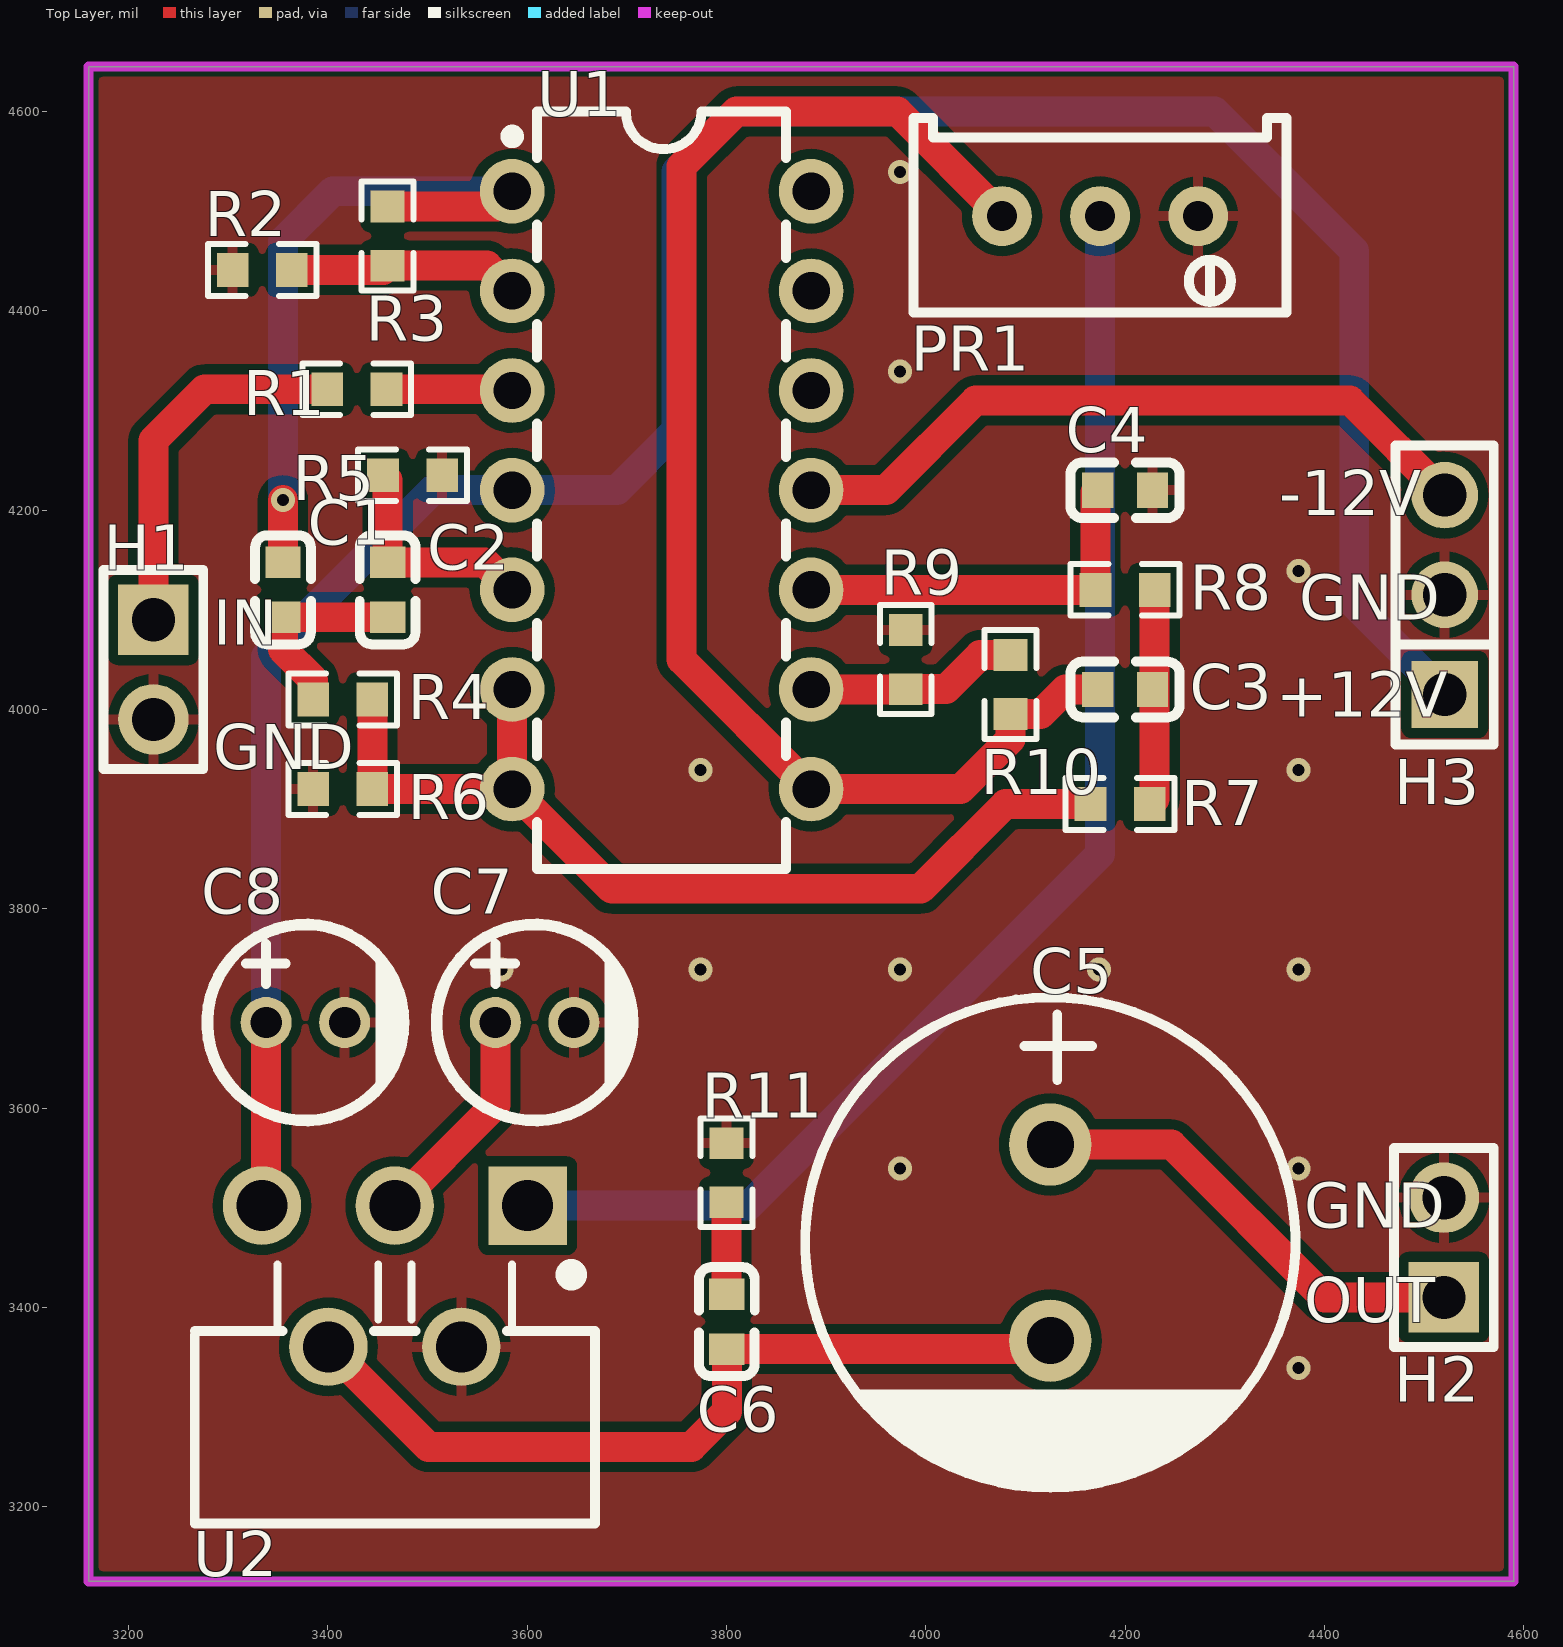
[diagram p0: Top Layer view]
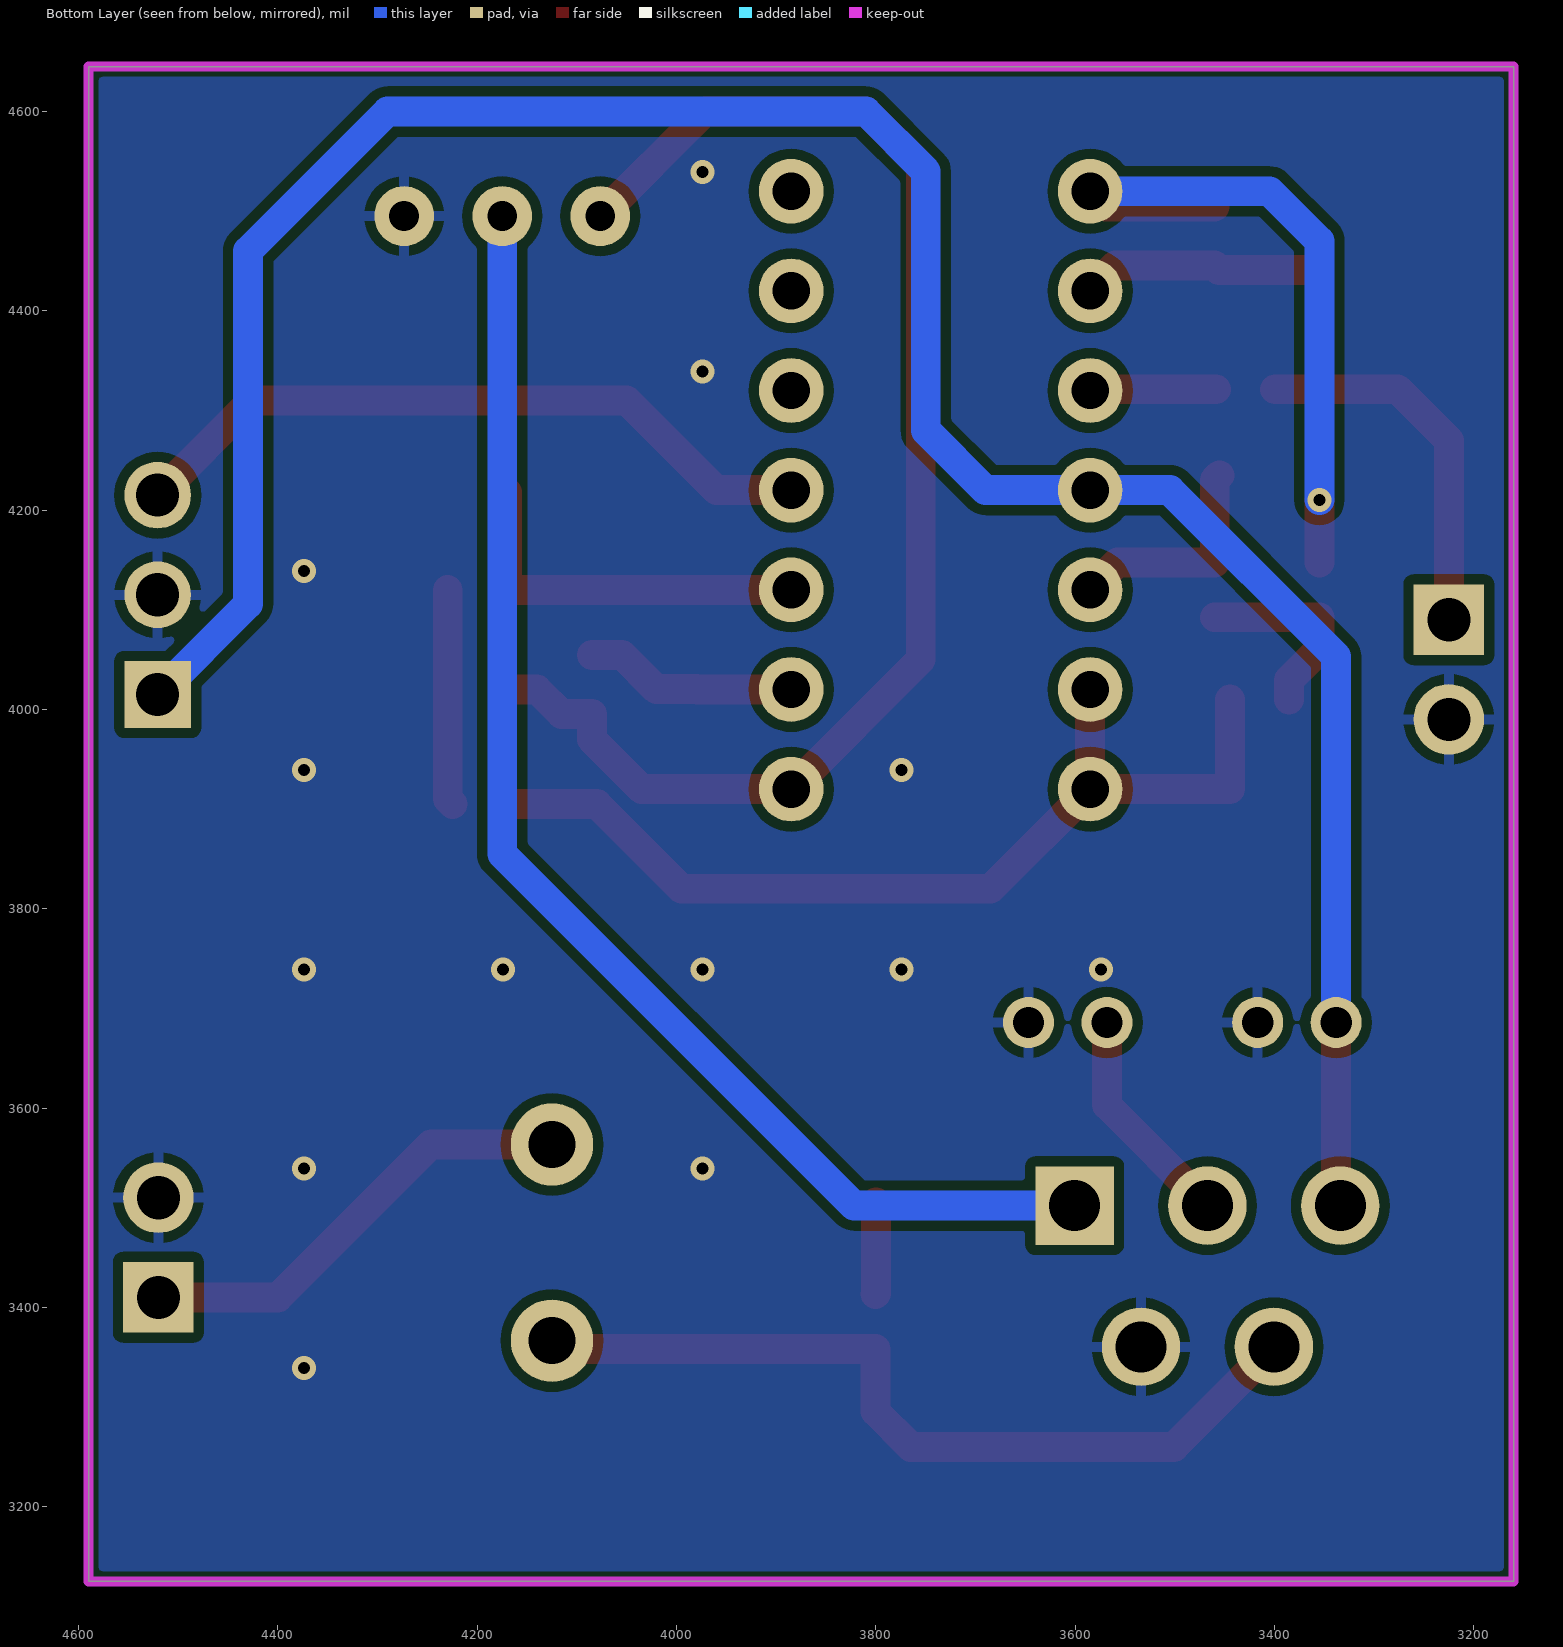
[diagram p1: Bottom Layer view, seen from below]
# Altium PCB MISC49872.pcbdoc
Units mil, origin at the board's own origin, x right, y up, seen from the top; angles counter-clockwise.
Board outline 1430 x 1520 mil, 2 copper layers (Top Layer, Bottom Layer), stack 62.206 mil thick; 25 components, 19 nets, 67 pads, 14 vias.

## Layer stack, top to bottom
Top Solder Mask Layer: solder mask 0.394, Dk 3.3
Top Layer: signal copper 1.379
Dielectric1: surface 59.449, FR4, Dk 4.5
Bottom Layer: signal copper 1.378
Bottom Solder Mask Layer: solder mask 0.394, Dk 3.3

## Board outline
3160,4645 3160,3125 4590,3125 4590,4645

## Design rules (kind name [scope] priority, off if disabled: settings)
BoardOutlineClearance copperThickness2oz_1 [All] p2 off: genericclearance=7.99 ignorepadtopadclearanceinfootprint=FALSE except(0: Arc-SplitContinuation Track-SplitContinuation SMDPad-SplitContinuation THPad-SplitContinuation Via-SplitContinuation Fill-SplitContinuation Region-SplitContinuation Poly-SplitContinuation Text-SplitContinuation Hole-SplitContinuation; 5.98: Arc-CutoutEdge SMDPad-CutoutEdge THPad-CutoutEdge Via-CutoutEdge Fill-CutoutEdge Region-CutoutEdge Text-CutoutEdge; 6.93: Hole-OutlineEdge Hole-CutoutEdge; 10: Poly-OutlineEdge Poly-CutoutEdge; 11.81: Arc-OutlineEdge Track-OutlineEdge SMDPad-OutlineEdge THPad-OutlineEdge Via-OutlineEdge Fill-OutlineEdge Region-OutlineEdge Text-OutlineEdge Track-CutoutEdge)
BoardOutlineClearance copperThickness1oz_1 [All] p4: genericclearance=4.02 ignorepadtopadclearanceinfootprint=FALSE except(0: Arc-SplitContinuation Track-SplitContinuation SMDPad-SplitContinuation THPad-SplitContinuation Via-SplitContinuation Fill-SplitContinuation Region-SplitContinuation Poly-SplitContinuation Text-SplitContinuation Hole-SplitContinuation; 6: SMDPad-CutoutEdge THPad-CutoutEdge Via-CutoutEdge Fill-CutoutEdge Region-CutoutEdge Text-CutoutEdge; 6.93: Hole-OutlineEdge Hole-CutoutEdge; 10: Poly-OutlineEdge Poly-CutoutEdge; 11.8: Arc-OutlineEdge Track-OutlineEdge SMDPad-OutlineEdge THPad-OutlineEdge Via-OutlineEdge Fill-OutlineEdge Region-OutlineEdge Text-OutlineEdge; 11.81: Arc-CutoutEdge Track-CutoutEdge)
Clearance copperThickness2oz [All] p1 off: gap=7.99 ignorepadtopadclearanceinfootprint=FALSE except(5.98: SMDPad-Track SMDPad-SMDPad THPad-Track SMDPad-THPad THPad-THPad Track-Via SMDPad-Via THPad-Via Via-Via Fill-Track Region-Track Fill-SMDPad Region-SMDPad Fill-THPad Region-THPad Fill-Via Region-Via Fill-Fill Fill-Region Region-Region Arc-Track Arc-SMDPad Arc-THPad Arc-Via Fill-Arc Region-Arc Arc-Arc Text-Track SMDPad-Text Text-THPad Text-Via Fill-Text Region-Text Arc-Text Text-Text; 6.93: Hole-Track Hole-SMDPad Hole-THPad Hole-Via Fill-Hole Region-Hole Hole-Arc Hole-Text; 10: Poly-Track Poly-SMDPad Poly-THPad Poly-Via Poly-Fill Poly-Region Poly-Poly Poly-Arc Poly-Text Poly-Hole)
Clearance copperThickness1oz [All] p3: gap=4.02 ignorepadtopadclearanceinfootprint=FALSE except(5.98: SMDPad-Track SMDPad-SMDPad THPad-Track SMDPad-THPad THPad-THPad Track-Via SMDPad-Via THPad-Via Via-Via Fill-Track Region-Track Fill-SMDPad Region-SMDPad Fill-THPad Region-THPad Fill-Via Region-Via Fill-Fill Fill-Region Region-Region; 6: Arc-Track Arc-SMDPad Arc-THPad Arc-Via Fill-Arc Region-Arc Arc-Arc Text-Track SMDPad-Text Text-THPad Text-Via Fill-Text Region-Text Arc-Text Text-Text; 6.93: Hole-Track Hole-SMDPad Hole-THPad Hole-Via Fill-Hole Region-Hole Hole-Arc Hole-Text; 10: Poly-Track Poly-SMDPad Poly-THPad Poly-Via Poly-Fill Poly-Region Poly-Poly Poly-Arc Poly-Text Poly-Hole)
Creepage creepage [All] p1: checkdistance=0 ignoreinternallayers=TRUE applytopolygonpour=TRUE
DiffPairsRouting differentialPair [All] p1: maxlimit=6 minlimit=6 mostfreqgap=6 toplayer_minwidth=5 toplayer_prefwidth=10 toplayer_maxwidth=100 toplayer_mingap=6 toplayer_prefgap=6 toplayer_maxgap=6 bottomlayer_minwidth=5 bottomlayer_prefwidth=10 bottomlayer_maxwidth=100 bottomlayer_mingap=6 bottomlayer_prefgap=6 bottomlayer_maxgap=6 maxuncoupledlength=10
HoleToHoleClearance otherClearance [All] p1: gap=11.81 allowstackedmicrovias=TRUE
Length netLength [All] p1: minlimit=0 maxlimit=0
MatchedLengths netLengthTolerance [All] p1: tolerance=1000
PasteMaskExpansion pasteMaskExpansion [All] p1: expansion=0
PlaneConnect innerPlane [All] p1: planeconnectstyle=Relief reliefexpansion=20 reliefentries=4 reliefconductorwidth=10 reliefairgap=10
PolygonConnect copperRegion [(InNet('GND'))] p1: connectstyle=Relief reliefconductorwidth=10 reliefentries=4 polygonreliefangle="90 Angle" airgapwidth=10 via.connectstyle=Relief via.reliefconductorwidth=10 via.reliefentries=4 via.polygonreliefangle="90 Angle" via.airgapwidth=10
RoutingVias viaSize [All] p1: holewidth=12.01 width=24.02 viastyle="Through Hole" minholewidth=11.81 minwidth=19.68 maxholewidth=248.03 maxwidth=393.7
SolderMaskExpansion solderMaskExpansion [IsVia] p1: expansion=-1000 istentingtop=TRUE
SolderMaskExpansion solderMaskExpansion [All] p2: expansion=2 istentingtop=FALSE
Width copperThickness2oz_2 [All] p1 off: maxlimit=100 minlimit=8 preferedwidth=10
Width copperThickness1oz_2 [All] p2: maxlimit=100 minlimit=5 preferedwidth=10

## Components (designator, comment, footprint, x,y, rotation, side; value= is the part's Value field where it differs from the comment)
C1 "100nF" C0603 3355,4120 r270 top
C2 "100nF" C0603 3460,4120 r90 top
C3 "10nF" C0603 4200,4020 r180 top
C4 "10nF" C0603 4200,4220 r0 top
C5 "1000uF" CAP-TH_BD12.5-P5.00-D0.6-FD 4125,3465 r270 top
C6 "0.051UF" C0603 3800.46,3385.61 r270 top
C7 "10uF" CAP-TH_BD5.0-P2.00-D0.8-FD-10UF50VC110GL 3607.49,3685.8 r0 top
C8 "10uF" CAP-TH_BD5.0-P2.00-D0.8-FD-10UF50VC110GL 3377.49,3685.8 r0 top
H1 "" HDR-TH_2P-P2.54-V-M-1 3225,4040 r270 top
H2 "" HDR-TH_2P-P2.54-V-M-1 4520,3460 r90 top
H3 "" HDR-TH_3P-P2.54-V-M 4520.79,4115 r90 top
PR1 "10kΩ" R_3296 4175,4490 r180 top
R1 "9.1" R0603 3429.18,4321.32 r0 top
R2 "10K" R0603 3334.18,4440.98 r0 top
R3 "100K" R0603 3460,4475 r90 top
R4 "15K" R0603 3415,4010 r0 top
R5 "15K" R0603 3485,4235 r0 top
R6 "15K" R0603 3415,3920 r180 top
R7 "15K" R0603 4195,3905 r0 top
R8 "15K" R0603 4200,4120 r180 top
R9 "100K" R0603 3980,4050 r270 top
R10 "27K" R0603 4085,4025 r270 top
R11 "10" R0603 3800,3535 r270 top
U1 "LM324N/PB" PDIP-14_L19.2-W6.6-P2.54-LS7.6-BL 3735,4220 r270 top
U2 "TDA2030A(XBLW)" TO-220-5_L10.5-W15.5-P1.70-TL 3467.25,3431.2 r270 top

## Footprints (in the part's own frame and the unit in brackets; to place one, negate y for a bottom-side part, rotate by r counter-clockwise, add the part's x,y. Pads: shape width x height; smd on the part's side, far side on the other; paste and mask are expansions set on the pad)
C0603 [mm]
  rect 0.8x0.9 smd: 1(-0.7,0) 2(0.7,0)
  silkscreen extent -1.39,-0.71 1.39,0.71
CAP-TH_BD5.0-P2.00-D0.8-FD-10UF50VC110GL [mm]
  round 1.3 hole 0.8: 1(-1,0) 2(1,0)
  silkscreen extent -2.5,-2.5 2.5,2.5
CAP-TH_BD12.5-P5.00-D0.6-FD [mm]
  round 2.1 hole 1.2 paste+0 mask+0.05: 1(-2.5,0) 2(2.5,0)
  silkscreen extent -6.25,-6.25 6.25,6.25
HDR-TH_2P-P2.54-V-M-1 [mm]
  rect 1.8x1.8 hole 1.1: 1(-1.27,0)
  round 1.8 hole 1.1: 2(1.27,0)
  silkscreen extent -2.54,-1.27 2.54,1.27
HDR-TH_3P-P2.54-V-M [mm]
  rect 1.7x1.7 hole 1.1: 1(-2.54,0)
  round 1.7 hole 1.1: 2(0,0) 3(2.54,0)
  silkscreen extent -3.81,-1.25 3.81,1.25
PDIP-14_L19.2-W6.6-P2.54-LS7.6-BL [mm]
  round 1.65 hole 0.95: 1(-7.62,-3.81) 2(-5.08,-3.81) 3(-2.54,-3.81) 4(0,-3.81) 5(2.54,-3.81) 6(5.08,-3.81) 7(7.62,-3.81) 8(7.62,3.81) 9(5.08,3.81) 10(2.54,3.81) 11(0,3.81) 12(-2.54,3.81) 13(-5.08,3.81) 14(-7.62,3.81)
  silkscreen extent -9.65,-3.96 9.65,3.17
R0603 [mil]
  rect 31.75x34.02 smd paste-3937.01 mask+2: 1(-29.66,0) 2(29.66,0)
  silkscreen extent -55,-26 55,26
R_3296 [mil]
  round 60 hole 30 paste+0 mask+2: 1(-98.4,-5) 2(0,-5) 3(98.4,-5)
  silkscreen extent -187,-103 187,92
TO-220-5_L10.5-W15.5-P1.70-TL [mm]
  rect 2x2 hole 1.3: 1(-1.8,3.386)
  round 2 hole 1.3: 2(1.8,1.694) 3(-1.8,0) 4(1.799,-1.694) 5(-1.8,-3.386)
  silkscreen extent -0.3,-5.1 6.3,5.1

## Via types
v1: diameter 24.02, hole 12, Top Layer to Bottom Layer, 14 vias

## Nets (pads, with @x,y where several pads share a name; then routed paths per layer and width w, separated by ;. In a path a pad name is that pad's centre, name@x,y a point inside that pad or via, vN(x,y) a via of type N, cw(c..) or ccw(c..) an arc to the next point about the centre after c; other vN are vias at no path point)
12V: C8.1 H3.1 U1.4 U2.5 | length 2564.1
  Top Layer w30: U2.5 3338.12,3506.22 C8.1
  Bottom Layer w30: C8.1 3338.12,4053.12 3505,4220 U1.4 3690,4220 3750,4280 3750,4540 3810,4600 4290,4600 4430,4460 4430,4105.79 H3.1
$1N1: R1.2 U1.3 | length 126.7
  Top Layer w30: R1.2 3583.69,4321.32 U1.3
$1N4: H1.1 R1.1 | length 375.8
  Top Layer w30: H1.1 3225,4270 3276.32,4321.32 R1.1
$1N8: R2.2 R3.1 U1.2 | length 233.5
  Top Layer w30: R2.2 3455.64,4440.98 R3.1 3559.67,4445.34 U1.2
$1N10: C1.1 R3.2 U1.1 | length 704.5
  Top Layer w30: C1.1 v1(3355,4210) ; R3.2 3569.66,4504.66 U1.1
  Bottom Layer w30: v1(3355,4210) 3355,4470 3405,4520 U1.1
$1N11: C2.2 R5.1 U1.5 | length 225.8
  Top Layer w30: R5.1 3460,4230.34 C2.2 3557.45,4147.56 U1.5
$1N13: C1.2 C2.1 R4.1 | length 200
  Top Layer w30: R4.1 3385.34,4029.66 3355,4060 C1.2 C2.1
$1N18: R4.2 R6.1 R7.1 U1.6 U1.7 | length 987.3
  Top Layer w30: R4.2 R6.1 U1.7 ; U1.6 U1.7 ; R7.1 4080,3905 3995,3820 3685.01,3820 U1.7
$1N19: C3.1 R7.2 R8.1 | length 217.1
  Top Layer w30: R7.2 4229.66,3910 R8.1
$1N20: C4.1 R8.2 U1.10 | length 386.2
  Top Layer w30: U1.10 R8.2 4170.34,4217.9 C4.1
$1N25: C3.2 PR1.3 R10.2 U1.8 | length 1410.4
  Top Layer w30: PR1.3 3971.6,4600 3810,4600 3755,4545 3755,4050.01 U1.8 4035,3920 4085,3970 R10.2 4115.34,3995.34 4140,4020 C3.2
$1N26: R9.2 R10.1 U1.9 | length 214.4
  Top Layer w30: U1.9 3979.66,4020 R9.2 4020.34,4020.34 4054.66,4054.66 R10.1
$1N28: PR1.2 U2.1 | length 1360.6
  Bottom Layer w30: U2.1 3822.06,3502.06 4175,3855 PR1.2
$1N34: C5.2 C6.2 U2.4 | length 846.8
  Top Layer w30: U2.4 3500.91,3260 3765,3260 3800.46,3295.46 C6.2 4116.47,3358.05 C5.2
$1N35: C6.1 R11.2 | length 92.4
  Top Layer w30: R11.2 3800,3413.62 C6.1
$1N37: C5.1 H2.1 | length 458.6
  Top Layer w30: C5.1 4246.57,3563.43 4400,3410 H2.1
$1N38: C7.1 U2.3 | length 225.5
  Top Layer w30: U2.3 3568.12,3602.92 C7.1
-12V: H3.3 U1.11 | length 712.4
  Top Layer w30: U1.11 3960,4220 4050,4310 4425.79,4310 H3.3
GND: C4.2 C7.2 C8.2 H1.2 H2.2 H3.2 PR1.1 R2.1 R5.2 R6.2 R9.1 R11.1 U2.2
  other v1: 4374.1,3339.1 3974.1,3539.1 4374.1,3539.1 3574.1,3739.1 3774.1,3739.1 3974.1,3739.1 4174.1,3739.1 4374.1,3739.1 3774.1,3939.1 4374.1,3939.1 4374.1,4139.1 3974.1,4339.1 3974.1,4539.1
pads on no net: U1.12 U1.13 U1.14

## Polygon pours and split planes (outlines as drawn)
GND on Top Layer (solid, remove dead copper, pour order 0): 3000,4715 3000,3000 4835,3000 4835,4715
GND on Bottom Layer (solid, remove dead copper, pour order 2): 3070,4715 3070,3070 4840,3070 4840,4715

## Keep-outs
Board Outline Layer:
  the board outline again, w10

## Silkscreen, mask and mechanical layers (free items; w line width, h text height)
Top Silkscreen Layer:
  text "-12V" at 4355,4195 h45
  text "GND" at 4375,4090 h45
  text "IN" at 3285,4065 h45
  text "+12V" at 4351.95,3992.5 h45
  text "GND" at 3285,3940 h45
  text "GND" at 4380,3480 h45
  text "OUT" at 4380,3385 h45